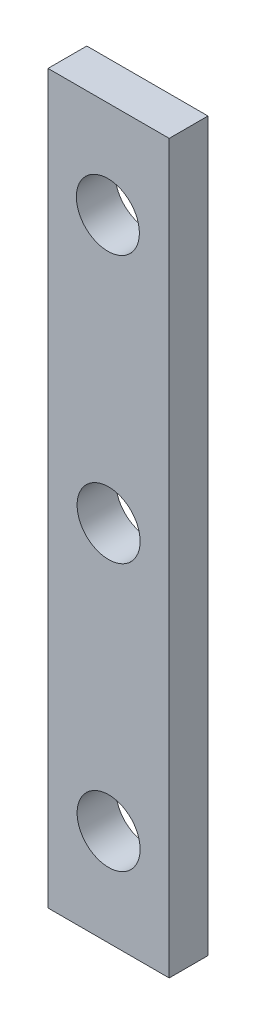
from build123d import *

# Parameters (mm, degrees)
SKETCH_1_W      = 25
SKETCH_1_H      = 150
SKETCH_1_R      = 6.5
EXTRUDE_1_DEPTH = 8


with BuildPart() as part:
    # 草图1 → 凸台-拉伸1 (new body)
    with BuildSketch(Plane.XY):
        Rectangle(SKETCH_1_W, SKETCH_1_H)
        with Locations((-0.153888597, 54.999784711)):
            Circle(SKETCH_1_R, mode=Mode.SUBTRACT)
        Circle(SKETCH_1_R, mode=Mode.SUBTRACT)
        with Locations((0, -55)):
            Circle(SKETCH_1_R, mode=Mode.SUBTRACT)
    extrude(amount=EXTRUDE_1_DEPTH)


solid = part.part
